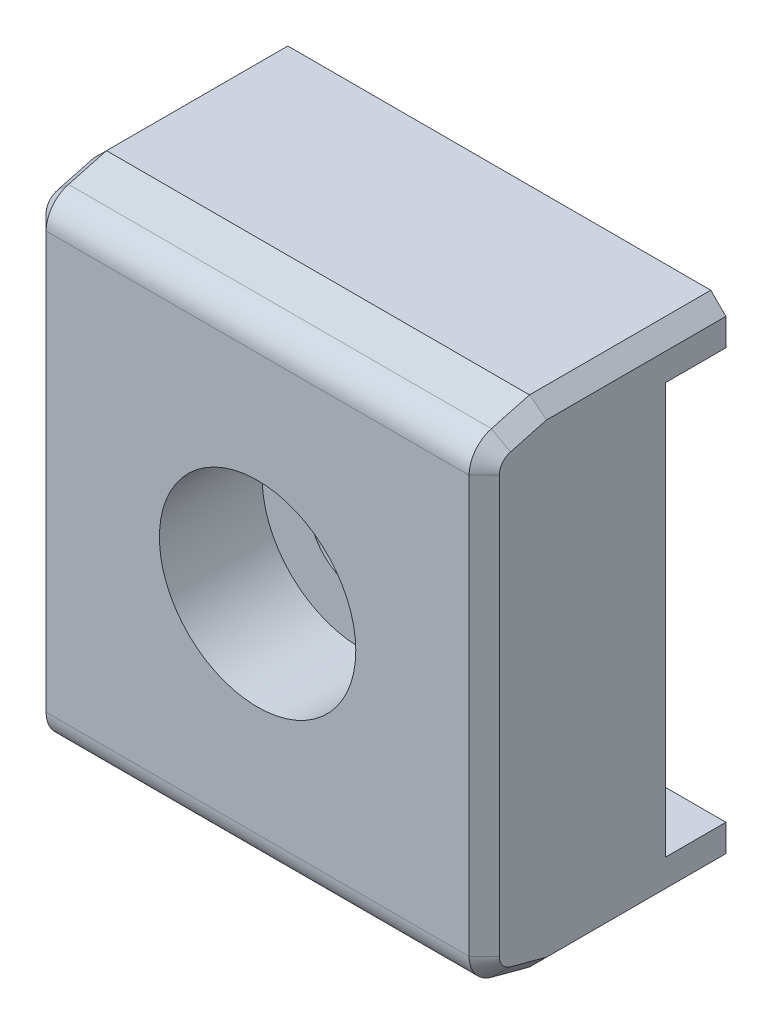
SolidWorks part; units mm, degrees
material "PEEK"
ref_plane "前视基准面" through (0, 0, 0) normal (0, 0, 1) x (1, 0, 0)
ref_plane "上视基准面" through (0, 0, 0) normal (0, 1, 0) x (1, 0, 0)
ref_plane "右视基准面" through (0, 0, 0) normal (1, 0, 0) x (0, 0, -1)
sketch "草图2" plane through (-7.5, 0, 0) normal (-1, 0, 0) x (0, 0, 1)
  line L0 (-6, -6.8) -> (-8, -6.8)
  line L2 (-8, -6.8) -> (-8, -8.2)
  line L3 (-8, -8.2) -> (-2, -8.2)
  line L4 (-2, -8.2) -> (-0.7412, -7.8627)
  line L5 (0, -6.8968) -> (0, 6.8968)
  line L6 (-6, 6.8) -> (-6, -6.8)
  line L7 (-6, 6.8) -> (-8, 6.8)
  line L12 (-2, 8.2) -> (-0.7412, 7.8627)
  line L13 (-8, 8.2) -> (-2, 8.2)
  line L14 (-8, 7.7) -> (-8, 8.2)
  line L15 (-8, 6.8) -> (-8, 7.7)
  arc A2 (-0.7412, -7.8627) -> (0, -6.8968) centre (-1, -6.8968) ccw
  arc A3 (0, 6.8968) -> (-0.7412, 7.8627) centre (-1, 6.8968) ccw
extrude "凸台-拉伸1" add sketch "草图2" against normal up to surface (15 mm away)
chamfer "倒角1" distance 0.5 angle 45 14 edges at (-7.5, -8.0314, -1.3706) (-7.5, 8.0314, -1.3706) (-7.5, -7.5055, -0.2066) (-7.5, 7.5055, -0.2066) (-7.5, 0, 0) (7.5, 8.0314, -1.3706) (7.5, -8.0314, -1.3706) (7.5, 7.5055, -0.2066) (7.5, -7.5055, -0.2066) (7.5, 0, 0) (-7.5, 8.2, -5) (7.5, 8.2, -5) (7.5, -8.2, -5) (-7.5, -8.2, -5)
hole_wizard "M3 六角凹头螺钉的柱形沉头孔1" positions "草图3" profile "草图4" counterbore size "M3" standard "ISO"
sketch "草图3" plane through (0, 0, 0) normal (0, 0, 1) x (1, 0, 0)
  point P0 (0, 0)
sketch "草图4" plane through (0, 0, 0) normal (1, 0, 0) x (0, -1, 0)
  line L0 (0, 0) -> (0, 11.0215)
  line L1 (0, 11.0215) -> (1.7, 10)
  line L2 (1.7, 10) -> (1.7, 3.4)
  line L3 (1.7, 3.4) -> (3.25, 3.4)
  line L4 (3.25, 3.4) -> (3.25, 0)
  line L5 (3.25, 0) -> (0, 0)
  line L10 (0, 11.0215) -> (-1.7, 10) construction
  line L11 (0, -6.35) -> (0, 107.95) construction
  dimension "孔直径" = 3.4
  dimension "孔深度" = 10
  dimension "柱形沉头孔直径" = 6.5
  dimension "柱形沉头孔深度" = 3.4
  dimension "导头角度" = 118
